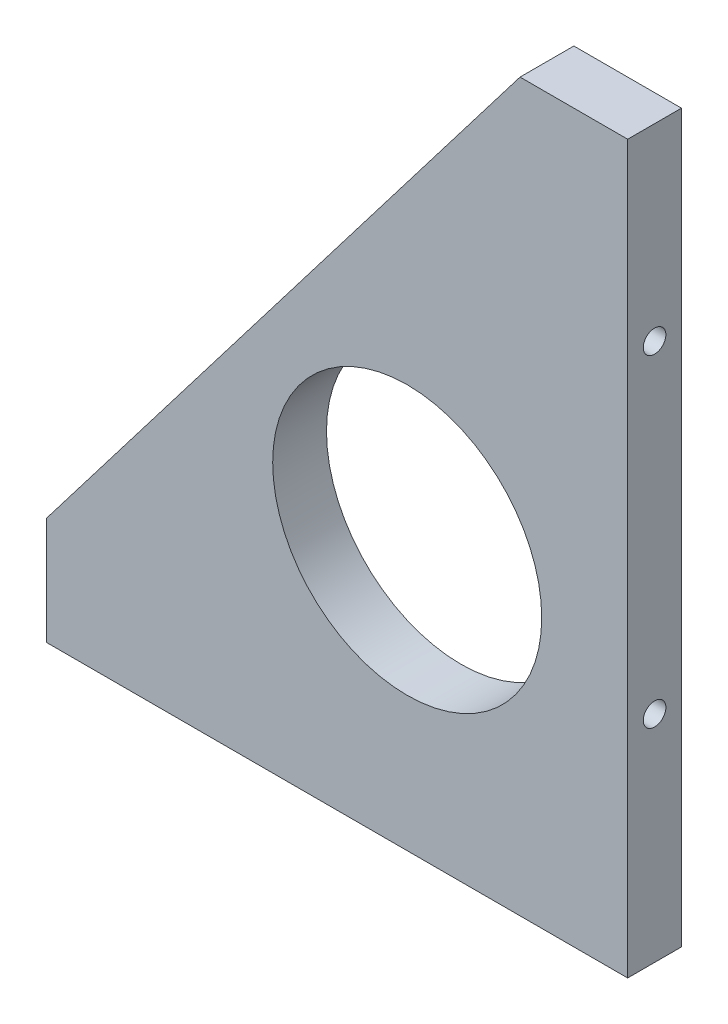
from build123d import *

# Parameters (mm, degrees)
SKETCH_1_W             = 108
SKETCH_1_H             = 135
EXTRUDE_1_DEPTH        = 10
CUT_EXTRUDE_1_REACH    = 89.019
HOLE_WIZARD_M5_1_D     = 4.2
HOLE_WIZARD_M5_1_DEPTH = 12.4
HOLE_WIZARD_M5_1_TIP   = 1.2618073
HOLE_WIZARD_M5_2_D     = 4.2
HOLE_WIZARD_M5_2_DEPTH = 12.4
HOLE_WIZARD_M5_2_TIP   = 1.2618073
CUT_EXTRUDE_2_REACH    = 89.019
SKETCH_7_R             = 25


with BuildPart() as part:
    # 草图1 → 凸台-拉伸1 (new body)
    with BuildSketch(Plane.XY):
        Rectangle(SKETCH_1_W, SKETCH_1_H)
    extrude(amount=EXTRUDE_1_DEPTH)

    # 草图2 → 切除-拉伸1 (cut, up to next)
    with BuildSketch(Plane.XY.offset(10), mode=Mode.PRIVATE) as cut_extrude_1_sk1:
        Polygon((34, 67.5), (-54, 67.5), (-54, -47.5), align=None)
    cut_extrude_1_tool1 = extrude(cut_extrude_1_sk1.sketch, amount=-CUT_EXTRUDE_1_REACH, mode=Mode.PRIVATE) & part.part
    add(cut_extrude_1_tool1.solids().sort_by_distance((-24.666667, 29.166667, 10))[0], mode=Mode.SUBTRACT)

    # M5 螺纹孔1
    with Locations(Plane(origin=(0, -67.5, 0), x_dir=(-1, 0, 0), z_dir=(0, -1, 0))):
        with Locations((-24, -5), (26, -5)):
            Hole(HOLE_WIZARD_M5_1_D / 2, depth=HOLE_WIZARD_M5_1_DEPTH)
            with Locations((0, 0, -(HOLE_WIZARD_M5_1_DEPTH + HOLE_WIZARD_M5_1_TIP / 2))):  # 118° drill point
                Cone(0, HOLE_WIZARD_M5_1_D / 2, HOLE_WIZARD_M5_1_TIP, mode=Mode.SUBTRACT)

    # M5 螺纹孔2
    with Locations(Plane(origin=(54, 0, 0), x_dir=(0, 0, -1), z_dir=(1, 0, 0))):
        with Locations((-5, -27.5), (-5, 32.5)):
            Hole(HOLE_WIZARD_M5_2_D / 2, depth=HOLE_WIZARD_M5_2_DEPTH)
            with Locations((0, 0, -(HOLE_WIZARD_M5_2_DEPTH + HOLE_WIZARD_M5_2_TIP / 2))):  # 118° drill point
                Cone(0, HOLE_WIZARD_M5_2_D / 2, HOLE_WIZARD_M5_2_TIP, mode=Mode.SUBTRACT)

    # 草图7 → 切除-拉伸2 (cut, up to next)
    with BuildSketch(Plane(origin=(0, 0, 0), x_dir=(-1, 0, 0), z_dir=(0, 0, -1)), mode=Mode.PRIVATE) as cut_extrude_2_sk1:
        with Locations((-13.028146721, -17.5)):
            Circle(SKETCH_7_R)
    cut_extrude_2_tool1 = extrude(cut_extrude_2_sk1.sketch, amount=-CUT_EXTRUDE_2_REACH, mode=Mode.PRIVATE) & part.part
    add(cut_extrude_2_tool1.solids().sort_by_distance((13.028147, -17.5, 0))[0], mode=Mode.SUBTRACT)


solid = part.part
